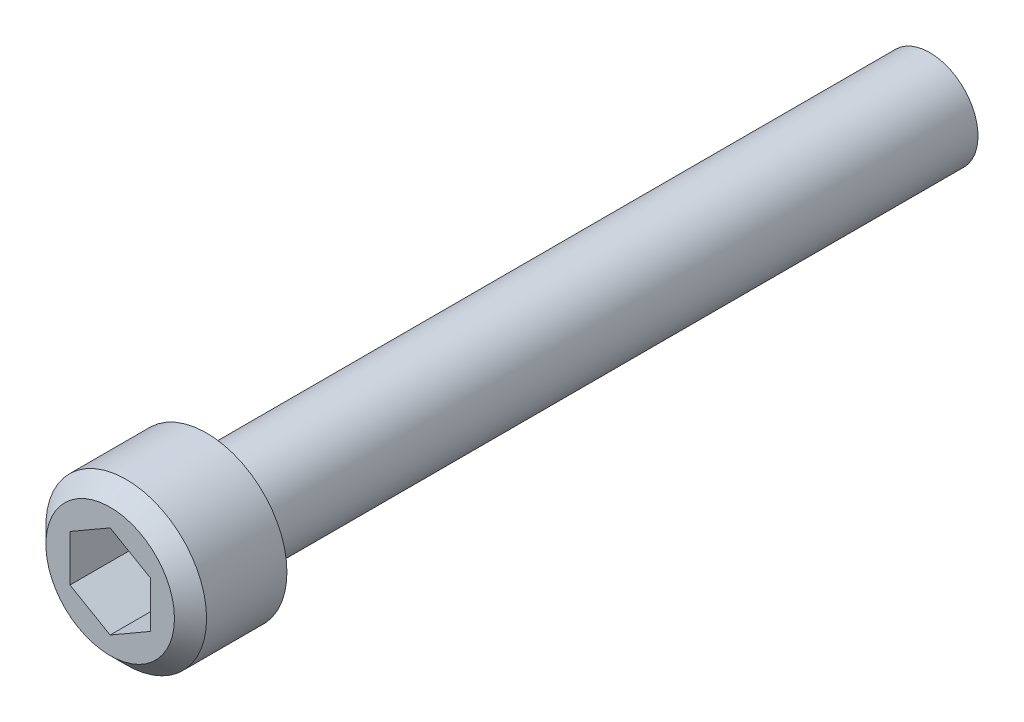
from build123d import *

# Parameters (mm, degrees)
SKETCH_1_R          = 5
EXTRUDE_1_DEPTH     = 6
CUT_EXTRUDE_1_DEPTH = 4
CHAMFER_1_SIZE      = 1
SKETCH_3_R          = 3
EXTRUDE_2_DEPTH     = 45


with BuildPart() as part:
    # 草图1 → 凸台-拉伸1 (new body)
    with BuildSketch(Plane.XY):
        Circle(SKETCH_1_R)
    extrude(amount=EXTRUDE_1_DEPTH)

    # 草图2 → 切除-拉伸1 (cut)
    with BuildSketch(Plane.XY.offset(6)):
        Polygon((0, 2.886751346), (-2.5, 1.443375673), (-2.5, -1.443375673), (0, -2.886751346), (2.5, -1.443375673), (2.5, 1.443375673), align=None)
    extrude(amount=-CUT_EXTRUDE_1_DEPTH, mode=Mode.SUBTRACT)

    # 倒角1
    chamfer_1_edges = [part.edges().sort_by_distance(p)[0] for p in [
        (-5, 0, 6),
    ]]
    chamfer(chamfer_1_edges, length=CHAMFER_1_SIZE)

    # 草图3 → 凸台-拉伸2 (add)
    with BuildSketch(Plane(origin=(0, 0, 0), x_dir=(-1, 0, 0), z_dir=(0, 0, -1))):
        with Locations(Location((0, 0, 0), (0, 0, 180))):
            Circle(SKETCH_3_R)
    extrude(amount=EXTRUDE_2_DEPTH)


solid = part.part
